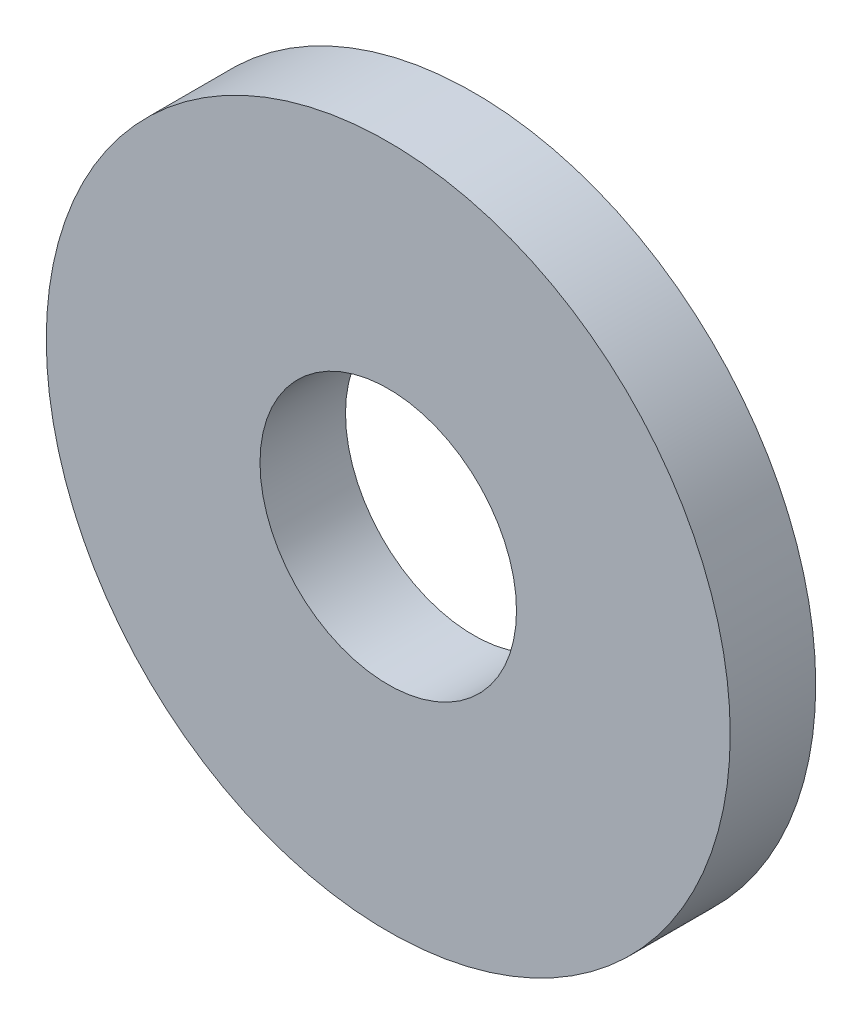
SolidWorks part; units mm, degrees
ref_plane "Front Plane" through (0, 0, 0) normal (0, 0, 1) x (1, 0, 0)
ref_plane "Top Plane" through (0, 0, 0) normal (0, 1, 0) x (1, 0, 0)
ref_plane "Right Plane" through (0, 0, 0) normal (1, 0, 0) x (0, 0, -1)
other "Configuration Table"
sketch "Sketch1" plane through (0, 0, 0) normal (0, 0, 1) x (1, 0, 0)
  circle A0 centre (0, 0) radius 1.5
  circle A1 centre (0, 0) radius 4
extrude "Boss-Extrude1" add sketch "Sketch1" along normal blind 1
